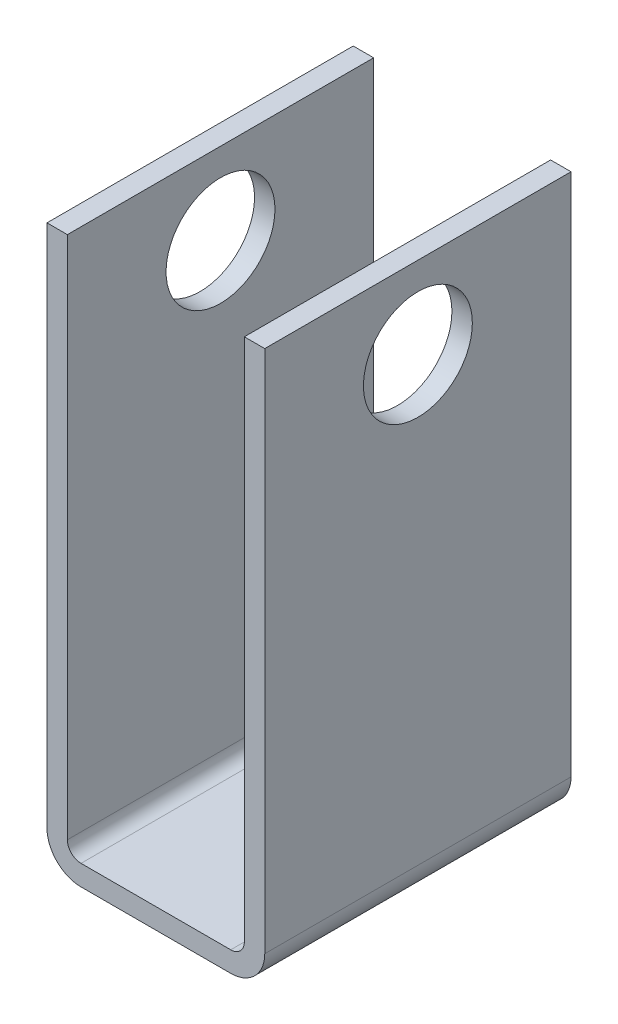
SolidWorks part; units mm, degrees
ref_plane "Front Plane" through (0, 0, 0) normal (0, 0, 1) x (1, 0, 0)
ref_plane "Top Plane" through (0, 0, 0) normal (0, 1, 0) x (1, 0, 0)
ref_plane "Right Plane" through (0, 0, 0) normal (1, 0, 0) x (0, 0, -1)
sketch "Sketch1" plane through (0, 0, 0) normal (0, 0, 1) x (1, 0, 0)
  line L0 (0, 0) -> (0, -77)
  line L1 (5, -82) -> (27, -82)
  line L2 (32, -77) -> (32, 0)
  line L3 (3, 0) -> (3, -77)
  line L4 (5, -79) -> (27, -79)
  line L5 (29, -77) -> (29, 0)
  line L6 (3, 0) -> (0, 0)
  line L7 (29, 0) -> (32, 0)
  arc A0 (27, -82) -> (32, -77) centre (27, -77) ccw
  arc A1 (0, -77) -> (5, -82) centre (5, -77) ccw
  arc A2 (3, -77) -> (5, -79) centre (5, -77) ccw
  arc A3 (27, -79) -> (29, -77) centre (27, -77) ccw
  point P8 (32, -82)
  point P11 (0, -82)
  dimension "D3" = 5
  dimension "D1" = 32
  dimension "D2" = 82
  dimension "D4" = 3
extrude "Boss-Extrude1" add sketch "Sketch1" along normal blind 45
sketch "Sketch2" plane through (32, 0, 0) normal (1, 0, 0) x (0, 0, -1)
  line L0 (0, -77) -> (0, 0) construction
  line L1 (-45, 0) -> (0, 0) construction
  circle A0 centre (-22.5, -12) radius 8
  dimension "D1" = 16
  dimension "D2" = 22.5
  dimension "D3" = 12
extrude "Cut-Extrude1" cut sketch "Sketch2" against normal through all
